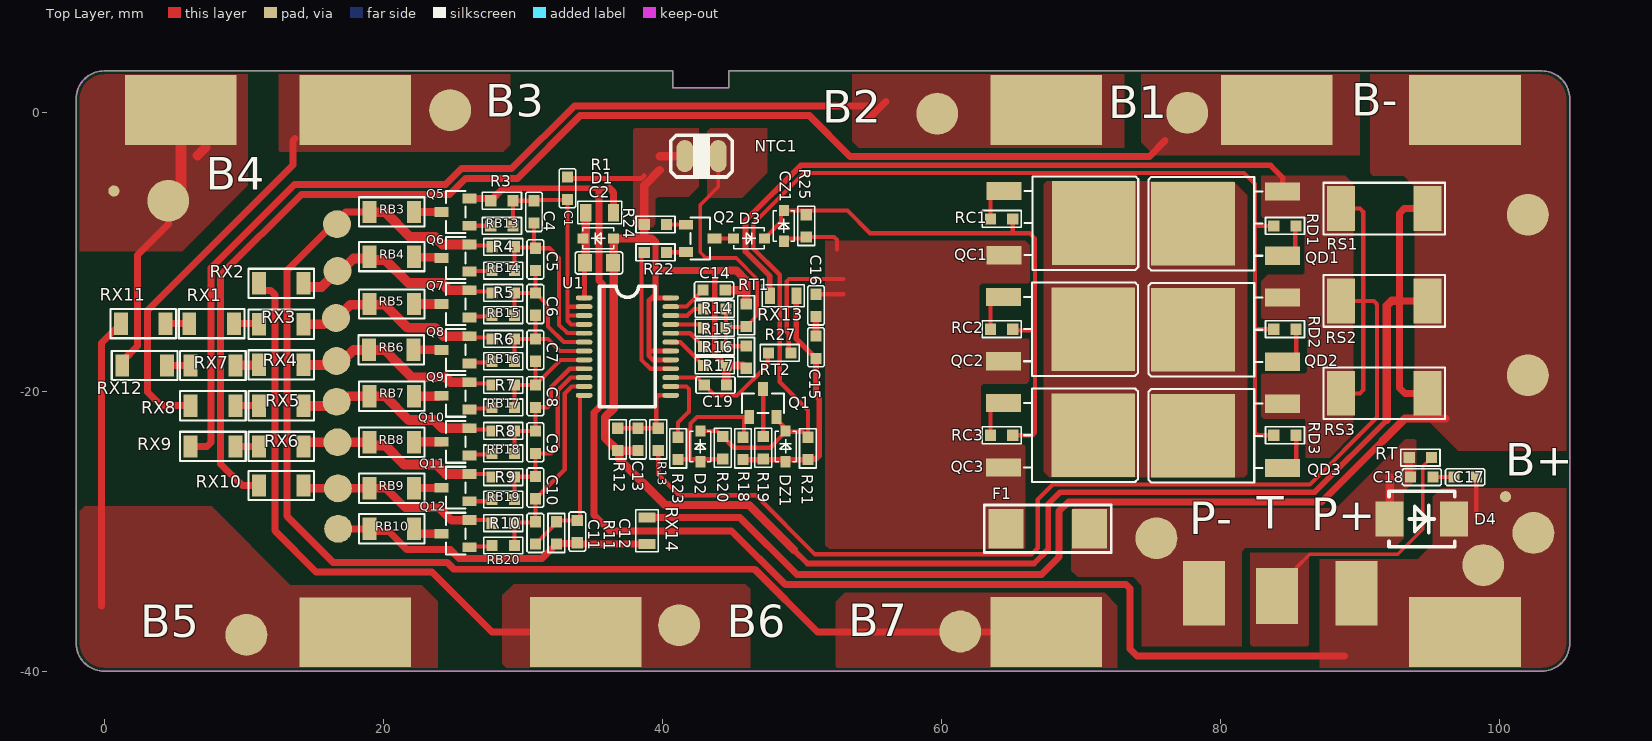
[diagram p0: Top Layer view]
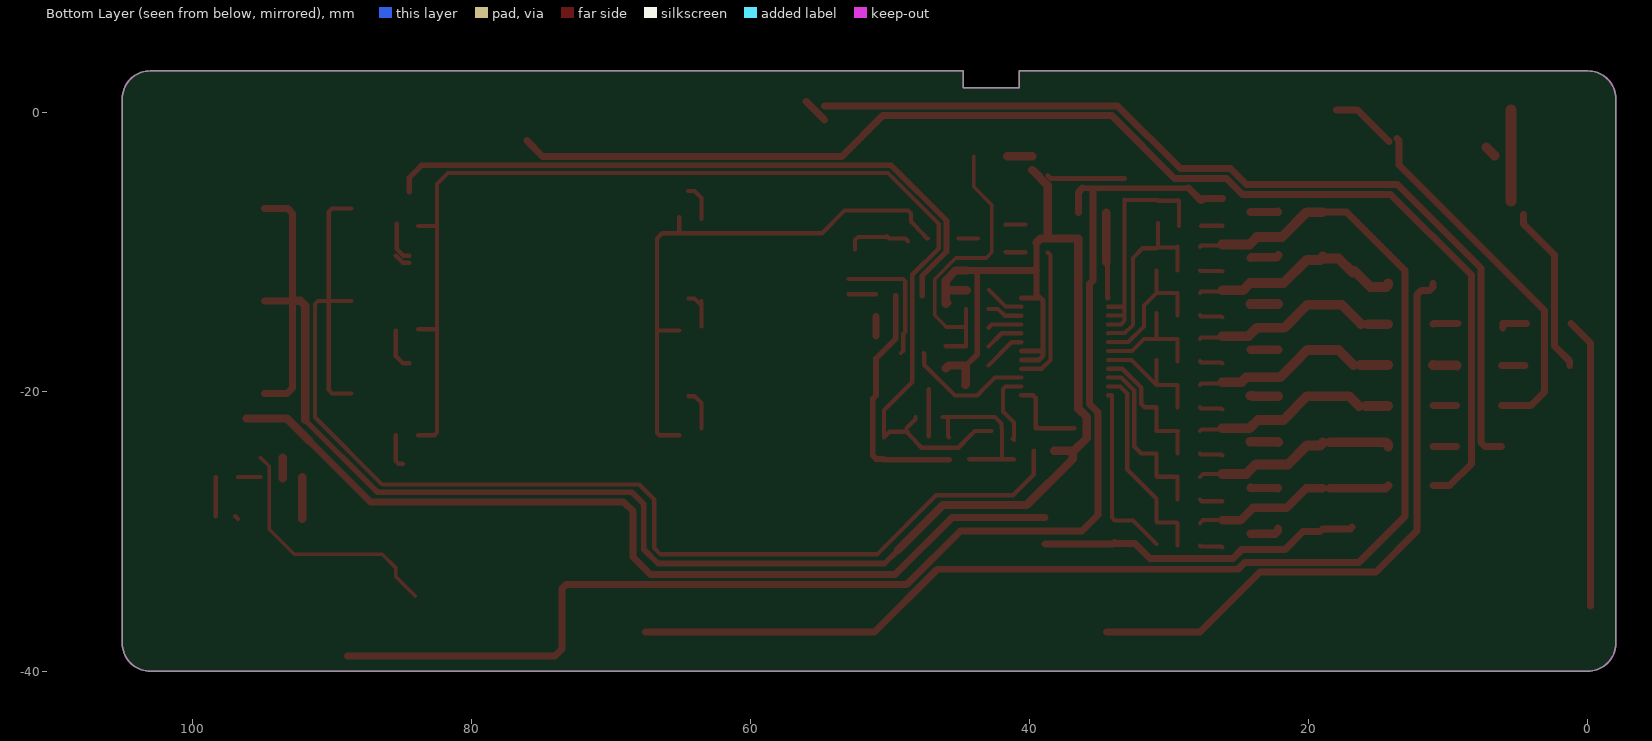
[diagram p1: Bottom Layer view, seen from below]
# Altium PCB MISC84401.PcbDoc
Units mm, origin at the board's own origin, x right, y up, seen from the top; angles counter-clockwise.
Board outline 107 x 43 mm, 2 copper layers (Top Layer, Bottom Layer); 122 components, 65 nets, 298 pads, 0 vias.
Unrouted connection lines stored in the file: 14.

## Layer stack, top to bottom (the 12.6 mil dielectric is the usual default, probably not edited)
Top Solder: solder mask 0.0102, Solder Resist, Dk 3.5
Top Layer: signal copper 0.0356
Dielectric 1: dielectric 0.32, FR-4, Dk 4.8
Bottom Layer: signal copper 0.0356
Bottom Solder: solder mask 0.0102, Solder Resist, Dk 3.5

## Board outline
-2,-38 -2,1 cw(c0,1) 0,3 40.751,3 40.751,1.8 44.751,1.8 44.751,3 103.001,3 cw(c103.001,1) 105.001,1 105.001,-38 cw(c103.001,-38) 103.001,-40 0,-40 cw(c0,-38)
board region "Default Layer Stack Region": -2,-38 -2,1 -2,1.197 -1.923,1.583 -1.772,1.947 -1.554,2.275 -1.275,2.554 -0.947,2.772 -0.583,2.923 -0.197,3 0,3 40.751,3 40.751,1.8 44.751,1.8 44.751,3 103.001,3 103.198,3 103.585,2.923 103.949,2.772 104.276,2.553 104.555,2.275 104.774,1.947 104.924,1.583 105.001,1.197 105.001,1 105.001,-38 105.001,-38.197 104.924,-38.584 104.774,-38.948 104.555,-39.275 104.276,-39.554 103.949,-39.773 103.585,-39.924 103.198,-40 103.001,-40 0,-40 -0.197,-40 -0.583,-39.924 -0.947,-39.773 -1.275,-39.554 -1.554,-39.275 -1.772,-38.948 -1.923,-38.584 -2,-38.197
board region "Layer Stack Region 1": -2,-38 -2,1 -2,1.197 -1.923,1.583 -1.772,1.947 -1.554,2.275 -1.275,2.554 -0.947,2.772 -0.583,2.923 -0.197,3 0,3 40.751,3 40.751,1.8 44.751,1.8 44.751,3 103.001,3 103.198,3 103.585,2.923 103.949,2.772 104.276,2.554 104.555,2.275 104.774,1.947 104.924,1.583 105.001,1.197 105.001,1 105.001,-38 105.001,-38.197 104.924,-38.584 104.774,-38.948 104.555,-39.275 104.276,-39.554 103.949,-39.773 103.585,-39.924 103.198,-40 103.001,-40 0,-40 -0.197,-40 -0.583,-39.924 -0.947,-39.773 -1.275,-39.554 -1.554,-39.275 -1.772,-38.948 -1.923,-38.584 -2,-38.197

## Design rules (kind name [scope] priority, off if disabled: settings)
Clearance [All] p1: gap=0.2 ignorepadtopadclearanceinfootprint=FALSE
ComponentClearance [All] p1: gap=0 collisioncheckmode=3 verticalgap=0 showdistances=FALSE
HoleToHoleClearance [All] p1: gap=0 allowstackedmicrovias=TRUE
MinimumSolderMaskSliver [All] p1: minsoldermaskwidth=0
PlaneConnect [All] p1: planeconnectstyle=Direct reliefexpansion=0.508 reliefentries=4 reliefconductorwidth=0.254 reliefairgap=0.254
PolygonConnect [All] p1: connectstyle=Direct reliefconductorwidth=0.254 reliefentries=4 polygonreliefangle="90 Angle" airgapwidth=0.254
RoutingVias [All] p1: holewidth=0.4 width=0.6 viastyle="Through Hole" minholewidth=0.4 minwidth=0.6 maxholewidth=0.4 maxwidth=0.6
SilkToSilkClearance [All] p1: silktosilkclearance=0
SilkToSolderMaskClearance [IsPad] p1: minsilkscreentomaskgap=0 clearancetoexposedcopper=TRUE
SolderMaskExpansion [All] p1: expansion=0.102 istentingtop=FALSE
SupplyNets "Schematic Supply Nets_1" [InNet('B-')] p1: voltage=0.000
SupplyNets "Schematic Supply Nets" [InNet('P-')] p2: voltage=0.000
Width [All] p1: maxlimit=1 minlimit=0.254 preferedwidth=0.254 minimp=50.000000 maximp=50.000000 favimp=50.000000
24 further rules are at their usual default settings.

## Components (designator, comment, footprint, x,y, rotation, side; value= is the part's Value field where it differs from the comment)
B1 "Pad" Pad10X8mm#1 84.001,0.2 r270 top locked
B2 "Pad" Pad10X8mm#2 67.501,-0.5 r270 top locked
B3 "Pad" Pad10X8mm#1 18,0.206 r270 top locked
B4 "Pad" Pad10X8mm#3 5.5,0.2 r270 top locked
B5 "Pad" Pad10X8mm#1 18,-37.2 r270 top locked
B6 "Pad" Pad10X8mm#3 34.5,-37.2 r270 top locked
B7 "Pad" Pad10X8mm#1 67.501,-37.194 r270 top locked
B+ "Pad" Pad10X8mm#1 97.501,-37.194 r270 top locked
B- "Pad" Pad10X8mm#3 97.501,0.2 r90 top locked
C1 "0.1uF" C0603A 33.2,-5.4 r270 top
C2 "1uF50V/0805" C0805A 35.45,-10.75 r180 top
C4 "0.1uF" C0603A 30.8,-7.1 r90 top
C5 "0.1uF" C0603A 30.9,-10.5 r90 top
C6 "0.1uF" C0603A 30.9,-13.7 r90 top
C7 "0.1uF" C0603A 30.9,-17 r90 top
C8 "0.1uF" C0603A 30.9,-20.3 r90 top
C9 "0.1uF" C0603A 30.9,-23.6 r90 top
C10 "0.1uF" C0603A 30.9,-26.85 r90 top
C11 "0.1uF" C0603A 30.9,-30.1 r90 top
C12 "1uF/NC*" C0603A 33.9,-30 r90 top
C13 "0.1uF" C0603A 38.25,-23.4 r90 top
C14 "0.1uF/NC*" C0603A 43.7,-12.7 r180 top
C15 "0.1uF" C0603A 51,-16.8 r270 top
C16 "0.1uF" C0603A 51,-13.8 r270 top
C17 "0.1uF" C0603A 97.5,-26.1 r0 top
C18 "0.1uF" C0603A 94.4,-26.1 r0 top
C19 "0.01uF/NC*" C0603A 43.8,-19.5 r0 top
CZ1 "15V" SOD323 48.7,-8.1 r270 top
D1 "56V" SOD323 35.4,-9 r0 top
D2 "1N4148SW/NC*" SOD323 42.72,-23.9 r270 top
D3 "1N4148SW" SOD323 46.2,-9 r180 top
D4 "RS3M" SMB(DO-214AA) 94.4,-29.1 r180 top
DZ1 "15V" SOD323 48.82,-23.9 r270 top
F1 "F2410 60V30A" F2410 67.6,-29.8 r0 top
NTC1 "10K B=3435" RT2.3X1.2-2 42.8,-3.1 r180 top
P+ "Pad" Pad10X8mm#4 82.122,-35.576 r270 top locked (schematic designator P+1)
P- "Pad" Pad10X8mm#5 86.327,-35.576 r270 top locked
Q1 "MMBT5401/N*" SOT23-3 47.2,-20.8 r0 top
Q2 "MMBT5401" SOT23-3 42.7,-9 r270 top
Q5 "MMBT5401" SOT23-3 25.189,-7.109 r90 top
Q6 "MMBT5401" SOT23-3 25.189,-10.401 r90 top
Q7 "MMBT5401" SOT23-3 25.189,-13.692 r90 top
Q8 "MMBT5401" SOT23-3 25.189,-16.984 r90 top
Q9 "MMBT5401" SOT23-3 25.189,-20.275 r90 top
Q10 "MMBT5401" SOT23-3 25.189,-23.567 r90 top
Q11 "MMBT5401" SOT23-3 25.189,-26.858 r90 top
Q12 "MMBT5401" SOT23-3 25.189,-30.15 r90 top
QC1 "TO-252 N MOS*" TO-252 67.687,-7.9 r270 top
QC2 "TO-252 N MOS*" TO-252 67.656,-15.5 r270 top
QC3 "TO-252 N MOS*" TO-252 67.656,-23.1 r270 top
QD1 "TO-252 N MOS*" TO-252 81.219,-7.939 r90 top
QD2 "TO-252 N MOS*" TO-252 81.219,-15.539 r90 top
QD3 "TO-252 N MOS*" TO-252 81.219,-23.139 r90 top
R1 "100R/1K*0805" R0805A#1 35.5,-7.15 r180 top
R3 "1K" R0603A 28.5,-6.3 r0 top
R4 "1K" R0603A 28.6,-9.6 r0 top
R5 "1K" R0603A 28.6,-12.9 r0 top
R6 "1K" R0603A 28.6,-16.2 r0 top
R7 "1K" R0603A 28.6,-19.5 r0 top
R8 "1K" R0603A 28.589,-22.792 r0 top
R9 "1K" R0603A 28.6,-26.1 r0 top
R10 "1K" R0603A 28.6,-29.4 r0 top
R11 "1K" R0603A 32.4,-30.1 r90 top
R12 "1K" R0603A 36.8,-23.4 r90 top
R13 "1K" R0603A 39.7,-23.4 r270 top
R14 "1K" R0603A 43.75,-14.05 r0 top
R15 "1K" R0603A 43.75,-15.4 r0 top
R16 "1K" R0603A 43.75,-16.75 r0 top
R17 "1K" R0603A 43.75,-18.1 r0 top
R18 "1K" R0603A 45.77,-24.042 r270 top
R19 "1K" R0603A 47.22,-24 r270 top
R20 "1K" R0603A 44.32,-24 r90 top
R21 "1K" R0603A 50.42,-24.042 r270 top
R22 "1K" R0603A 39.5,-10 r0 top
R23 "1K" R0603A 41.12,-24.042 r270 top
R24 "1K" R0603A 39.5,-8 r180 top
R25 "1K" R0603A 50.3,-8.1 r270 top
R27 "1K" R0603A 48.4,-17.2 r180 top
RB3 "51R" R1206A 20.6,-7.1 r0 top
RB4 "51R" R1206A 20.6,-10.3 r0 top
RB5 "51R" R1206A 20.6,-13.7 r0 top
RB6 "51R" R1206A 20.573,-16.984 r0 top
RB7 "51R" R1206A 20.6,-20.3 r0 top
RB8 "51R" R1206A 20.6,-23.6 r0 top
RB9 "51R" R1206A 20.6,-26.9 r0 top
RB10 "51R" R1206A 20.6,-29.8 r0 top
RB13 "1K" R0603A 28.5,-8.1 r0 top
RB14 "1K" R0603A 28.6,-11.3 r0 top
RB15 "1K" R0603A 28.6,-14.5 r0 top
RB16 "1K" R0603A 28.6,-17.8 r0 top
RB17 "1K" R0603A 28.6,-21.1 r0 top
RB18 "1K" R0603A 28.6,-24.4 r0 top
RB19 "1K" R0603A 28.6,-27.7 r0 top
RB20 "1K" R0603A 28.6,-31 r0 top
RC1 "1K" R0603A 64.3,-7.6 r0 top
RC2 "1K" R0603A 64.3,-15.5 r180 top
RC3 "1K" R0603A 64.3,-23.1 r180 top
RD1 "1K" R0603A 84.6,-8.1 r180 top
RD2 "1K" R0603A 84.6,-15.5 r180 top
RD3 "1K" R0603A 84.6,-23.1 r180 top
RS1 "R010" R2512L 91.7,-6.859 r180 top
RS2 "R010" R2512L 91.7,-13.48 r180 top
RS3 "R010" R2512L 91.7,-20.1 r180 top
RT "1K" R0603A 94.3,-24.7 r0 top
RT1 "1K" R0603A 46,-14.5 r90 top
RT2 "1K" R0603A 46,-17.5 r270 top
RX1 "1K" R1206A 7.7,-15.1 r180 top
RX2 "1K" R1206A 12.7,-12.22 r180 top
RX3 "1K" R1206A 12.7,-15.14 r180 top
RX4 "1K" R1206A 12.7,-18.06 r180 top
RX5 "1K" R1206A 12.7,-20.98 r180 top
RX6 "1K" R1206A 12.7,-23.9 r180 top
RX7 "1K" R1206A 7.8,-18.1 r180 top
RX8 "1K" R1206A 7.8,-20.98 r0 top
RX9 "1K" R1206A 7.8,-23.9 r0 top
RX10 "1K" R1206A 12.7,-26.7 r0 top
RX11 "1K" R1206A 2.8,-15.1 r180 top
RX12 "1K" R1206A 2.9,-18.1 r180 top
RX13 "1K" R0805A#2 48.65,-13.1 r180 top
RX14 "1K" R0805A#2 38.9,-29.95 r90 top
T "Pad" Pad10X8mm#6 84.019,-34.617 r90 top locked
U1 "CW1104/ERP2018" TSSOP-24(pin间距0.635mm) 37.491,-16.746 r0 top

## Footprints (in the part's own frame and the unit in brackets; to place one, negate y for a bottom-side part, rotate by r counter-clockwise, add the part's x,y. Pads: shape width x height; smd on the part's side, far side on the other; paste and mask are expansions set on the pad)
C0603A [mm] "贴片电容"
  rect 0.8x0.8 smd mask+0.08: 1(-0.8,0) 2(0.8,0)
  silkscreen extent -1.4,-0.6 1.4,0.6
C0805A [mm] "贴片电容"
  rect 1x1.25 smd: 1(-1,0)
  rect 1x1.25 smd mask+0.102: 2(1,0)
  silkscreen extent -1.7,-0.8 1.7,0.8
F2410 [mm] "贴片保险丝"
  rect 2.5x2.8 smd: 1(-3,0) 2(3,0)
  silkscreen extent -4.55,-1.7 4.55,1.7
Pad10X8mm#1 [mm]
  rect 5x8 smd: 1(0.006,0)
Pad10X8mm#2 [mm]
  rect 5x8 smd: 1(-0.7,0)
Pad10X8mm#3 [mm]
  rect 5x8 smd: 1(0,0)
Pad10X8mm#4 [mm]
  rect 4.6x3 smd: 1(-1.154,7.6)
Pad10X8mm#5 [mm]
  rect 4.6x3 smd: 1(-1.154,-7.524)
Pad10X8mm#6 [mm]
  rect 4x3 smd: 1(0,0)
R0603A [mm] "贴片电阻"
  rect 0.8x0.8 smd mask+0.08: 1(-0.8,0) 2(0.8,0)
  silkscreen extent -1.4,-0.6 1.4,0.6
R0805A#1 [mm] "贴片电阻"
  rect 0.8x1.25 smd paste+0 mask+0.08: 1(-1,0) 2(1,0)
  silkscreen extent -1.58,-0.8 1.58,0.8
R0805A#2 [mm] "贴片电阻"
  rect 0.7x1.2 smd paste+0 mask+0.08: 1(-0.95,0) 2(0.95,0)
  silkscreen extent -1.5,-0.8 1.5,0.8
R1206A [mm] "贴片电阻"
  rect 1x1.6 smd: 1(-1.6,0) 2(1.6,0)
  silkscreen extent -2.35,-1.05 2.35,1.05
R2512L [mm] "贴片电阻"
  rect 2x3.2 smd: 1(-3.1,0) 2(3.1,0)
  silkscreen extent -4.35,-1.85 4.35,1.85
RT2.3X1.2-2 [mm] "焊线NTC"
  oval 1.2x2.3 smd: 1(-1.2,0) 2(1.2,0)
  silkscreen extent -2.2,-1.55 2.2,1.5
SMB(DO-214AA) [mm] "贴片二极管"
  rect 2x2.5 smd: 1(-2.3,0) 2(2.3,0)
  silkscreen extent -2.35,-2 2.35,2
SOD323 [mm] "贴片二极管"
  rect 0.8x0.7 smd: 1(-1.1,0) 2(1.1,0)
  silkscreen extent -1.1,-0.75 1.1,0.75
SOT23-3 [mm] "贴片IC/MOS*"
  rect 0.7x1 smd: 1(-0.975,-1) 2(0.975,-1) 3(0,1.016)
  silkscreen extent -1.5,-0.7 1.5,0.7
TO-252 [mm]
  rect 1.3x2.5 smd: 1(-2.3,-3.212) 2(2.3,-3.212)
  rect 6x6 smd: 3(0,3.213)
  silkscreen extent -3.35,-1.75 3.35,6.4
TSSOP-24(pin间距0.635mm) [mm] "贴片IC"
  oval 1.2x0.35 smd: 1(-3.1,3.492) 1(-3.1,3.492) 2(-3.1,2.857) 3(-3.1,2.222) 4(-3.1,1.587) 5(-3.1,0.953) 6(-3.1,0.318) 7(-3.1,-0.318) 8(-3.1,-0.953) 9(-3.1,-1.587) 10(-3.1,-2.222) 11(-3.1,-2.858) 12(-3.1,-3.493) 13(3.1,-3.493) 13(3.1,-3.493) 14(3.1,-2.858) 15(3.1,-2.222) 16(3.1,-1.587) 17(3.1,-0.953) 18(3.1,-0.318) 19(3.1,0.318) 20(3.1,0.953) 21(3.1,1.587) 22(3.1,2.222) 23(3.1,2.857) 24(3.1,3.492)
  silkscreen extent -2,-4.33 2,4.33

## Part data
B1 B2 B3 B4 B5 B6 B7 B+ B- P+ P- T: "Connection pad (non-through-hole)"
C1 C2 C4 C5 C6 C7 C8 C9 C10 C11 C12 C13 C14 C15 C16 C17 C18 C19: library part CAP, "SMD capacitor"
CZ1 D1 DZ1: library part 5V6, "SMD Zener diode"
D2: library part 1N4148SW, "SMD diode"
D3 D4: "SMD diode"
F1: library part FUSE
NTC1: library part NTC, "SMD thermistor"
Q1: library part MMBT5401, "SMD transistor"
Q2 Q5 Q6 Q7 Q8 Q9 Q10 Q11 Q12: "SMD transistor"
QC1 QC2 QC3 QD1 QD2 QD3: library part "N MOS*", "SMD MOS"
R1 R3 R4 R5 R6 R7 R8 R9 R10 R11 R12 R13 R14 R15 R16 R17 R18 R19 R20 R21 R22 R23 R24 R25 R27 RB13 RB14 RB15 RB16 RB17 RB18 RB19 RB20 RC1 RC2 RC3 RD1 RD2 RD3 RT RT1 RT2 RX1 RX2 RX3 RX4 RX5 RX6 RX7 RX8 RX9 RX10 RX11 RX12 RX13 RX14: library part RES, "SMD resistor"
RB3 RB4 RB5 RB6 RB7 RB8 RB9 RB10: library part RES3, "Alloy SMD resistor"
RS1 RS2 RS3: library part RES2, "SMD alloy resistor"
U1: library part CW1104*, "Cellwise 7-10S battery protection IC"

## Free pads (board coordinates)
  round 0.8 smd: 2(0.7,-5.6) 2(100.4,-27.5)
  round 3 smd: 3(102,-18.8) 4(102,-7.3) 5(10.2,-37.4) 5(24.789,0.191) 5(59.689,-0.059) 5(61.339,-37.159) 5(77.6,0) 6(4.6,-6.3) 7(41.189,-36.709) 8(75.39,-30.48) 8(98.8,-32.4) 8(102.4,-30.1)
  rect 2.5x20 on Top Solder: 9(53.8,-20.7) 9(56.5,-20.7) 9(59.2,-20.7) 9(98.3,-13.8)
  round 2 smd: 10(16.61,-14.7) 10(16.64,-17.78) 10(16.66,-20.7) 10(16.69,-7.98) 10(16.72,-11.33) 10(16.75,-26.9) 10(16.77,-29.8) 11(16.725,-23.6)

## Nets (pads, with @x,y where several pads share a name; then routed paths per layer and width w, separated by ;. In a path a pad name is that pad's centre, name@x,y a point inside that pad or via, vN(x,y) a via of type N, cw(c..) or ccw(c..) an arc to the next point about the centre after c; other vN are vias at no path point)
B1: B1.1 pad.5@77.6,0 pad.10@16.75,-26.9 Q12.2 R10.1 RB9.1 RX10.1 RX10.2 | length 105.1
  Top Layer w0.3: Q12.2 27.575,-29.175 R10.1
  Top Layer w0.5: RX10.1 9.9,-26.7 8.35,-25.15 8.35,-11.63 14.138,-5.842 24.758,-5.842 25.9,-4.7 29.61,-4.7 34.11,-0.2 50.52,-0.2 53.44,-3.12 74.89,-3.12 76.02,-1.99
  Top Layer w0.6: RX10.2 14.5,-26.9 RB9.1@18.5,-26.9 ; RB9.1 20.193,-26.9 21.593,-28.3 24,-28.3 24.9,-29.2 26.164,-29.2 Q12.2
B2: B2.1 pad.5@59.689,-0.059 pad.11 Q11.2 R9.1 RB8.1 RX6.1 RX6.2 RX9.1 RX9.2 | length 83.8
  Top Layer w0.3: Q11.2 27.583,-25.883 R9.1
  Top Layer w0.5: RX9.1 7.357,-23.9 7.65,-23.607 7.65,-11.13 13.638,-5.142 24.458,-5.142 25.6,-4 29.2,-4 33.7,0.5 54.7,0.5 ; RX9.2 RX6.2 ; 54.7,-0.5 56,0.8
  Top Layer w0.7: RX6.1 14.3,-23.75 14.45,-23.6 RB8.1@18.5,-23.6 ; RB8.1 19,-23.69 19.15,-23.84 20.14,-23.84 21.5,-25.2 23.8,-25.2 24.483,-25.883 Q11.2
B3: B3.1 pad.5@24.789,0.191 pad.10@16.66,-20.7 Q10.2 R8.1 RB7.1 RX5.1 RX5.2 RX8.1 RX8.2 | length 46.7
  Top Layer w0.3: Q10.2 26.289,-22.692 27.689,-22.692 R8.1
  Top Layer w0.5: RX8.1 4.08,-20.98 3.1,-20 3.1,-14.173 13.537,-3.737 13.537,-1.983 13.68,-1.84 ; RX8.2 RX5.2 ; B3.1@14.25,-2.05 16.5,0.2 B3.1
  Top Layer w0.7: RX5.1 14.32,-21 pad.10@15.9,-21 ; pad.10@16.4,-21 17.1,-20.3 RB7.1 20.122,-20.3 21.822,-22 23.634,-22 24.226,-22.592 Q10.2
B4: B4.1 pad.2@0.7,-5.6 pad.6 pad.10@16.64,-17.78 Q9.2 R7.1 RB6.1 RX4.1 RX4.2 RX7.1 RX7.2 RX12.1 RX12.2 | length 37.4
  Top Layer w0.3: Q9.2 26.288,-19.4 27.7,-19.4 R7.1
  Top Layer w0.5: RX12.2 1.3,-17.8 2.4,-16.7 2.4,-10.176 4.6,-7.976 pad.6@4.6,-7.3 ; RX12.1 RX7.2
  Top Layer w0.7: 6.7,-3.05 7.279,-2.471 ; RX7.1 9.42,-18.08 11.08,-18.08 RX4.2 ; RX4.1 pad.10@16.3,-18.06 ; pad.10@16.8,-18.06 17.858,-17.002 20.113,-17.002 20.984,-17.873 22.061,-18.95 24.475,-18.95 24.825,-19.3 Q9.2
  Top Layer w0.8: pad.6@5.5,-6.3 B4.1
B5: B5.1 pad.5@10.2,-37.4 pad.10@16.61,-14.7 Q8.2 R6.1 RB5.1 RX1.1 RX1.2 RX3.1 RX3.2 RX11.1 RX11.2 | length 39.2
  Top Layer w0.3: Q8.2@26.18,-16 Q8.2 26.284,-16.104 27.704,-16.104 R6.1
  Top Layer w0.5: -0.2,-35.34 -0.2,-16.54 ; -0.2,-16.5 RX11.2 ; RX11.1 RX1.2 RX1.2@6.1,-15.4 ; RX1.1 11.06,-15.1 RX3.2
  Top Layer w0.7: RX3.1 pad.10@15.76,-15.14 ; pad.10@16.26,-15.14 17.651,-13.749 20.1,-13.749 21.751,-15.4 23.702,-15.4 24.302,-16 Q8.2@26.18,-16
B6: B6.1 pad.7 pad.10@16.72,-11.33 Q7.2 R5.1 RB4.1 RX2.1 RX2.2 | length 59.4
  Top Layer w0.3: Q7.2 26.28,-12.809 27.709,-12.809 R5.1
  Top Layer w0.5: RX2.2 11.1,-12.494 11.35,-12.744 11.937,-12.744 12.23,-13.036 12.23,-29.94 15.19,-32.9 23.5,-32.9 27.8,-37.2 B6.1
  Top Layer w0.7: RX2.1 14.3,-12.33 14.45,-12.48 15.57,-12.48 pad.10@16.72,-11.33 ; pad.10@16.845,-11.455 17.86,-10.44 18.86,-10.44 RB4.1 19,-10.39 19.15,-10.54 20.14,-10.54 21.8,-12.2 24.2,-12.2 24.717,-12.717 Q7.2
B7: B7.1 pad.5@61.339,-37.159 pad.10@16.69,-7.98 Q6.2 R4.1 RB3.1 | length 92.9
  Top Layer w0.3: Q6.2 26.276,-9.513 27.713,-9.513 R4.1
  Top Layer w0.5: RB3.1@19,-7.118 17.282,-7.118 13.1,-11.3 13.1,-28.9 16.4,-32.2 24.569,-32.2 25.069,-32.7 46.61,-32.7 51.11,-37.2 61.339,-37.2 B7.1
  Top Layer w0.7: RB3.1@19,-7.118 20.14,-7.118 21.922,-8.9 23.718,-8.9 24.243,-9.426 Q6.2
B+: B+.1 C17.2 D4.1 P+.1 pad.2@100.4,-27.5 pad.8@98.8,-32.4 pad.8@102.4,-30.1 Q5.2 R1.1 R3.1 | length 99.6
  Top Layer w0.3: D4.1 D4.1@96.9,-28.9 ; 98.3,-28.899 C17.2
  Top Layer w0.4: 28.6,-5.4 36.207,-5.4
  Top Layer w0.5: Q5.2 27.534,-6.134 R3.1 28.6,-5.4 ; 35.45,-5.45 35.45,-12 35.7,-12.25 35.7,-20.869 35.1,-21.469 35.1,-28.8 36.25,-29.95 44.96,-29.95 48.8,-33.79 73.207,-33.79 73.5,-34.083 73.5,-38.4 74,-38.9 88.872,-38.9 ; 36.207,-5.4 36.5,-5.693 R1.1
B-: B-.1 C1.1 C2.1 C12.1 C13.1 C14.1 C19.2 D1.2 NTC1.2 pad.3 pad.4 pad.10@16.77,-29.8 R11.1 R12.1 R17.2 R24.2 RB10.1 RS1.1 RS2.1 RS3.1 RT1.2 RT2.2 RX14.1 RX14.2 U1.17 U1.18 U1.24 | length 247.9
  Top Layer w0.35: C1.1@33.2,-4.7 38.5,-4.7 38.7,-4.5 ; 39.025,-13.459 39.025,-17.1 ; 39.255,-13.254 U1.24 ; U1.17 39.324,-17.699 39.025,-17.4 39.025,-17.1 ; U1.18 39.061,-17.064 39.025,-17.1
  Top Layer w0.4: 39.05,-13.459 39.255,-13.254 39.5,-13.009 39.5,-11.3 39.5,-9.3 ; 43.712,-11.3 43.75,-11.338 43.75,-17.316 44.033,-17.599 44.049,-17.599 R17.2 ; 49.4,-31.3 50.39,-32.29 66.62,-32.29 67.64,-31.27 67.64,-28.02 68.48,-27.18 86.72,-27.18 91.9,-22
  Top Layer w0.5: pad.10@16.9,-29.68 17.02,-29.8 RB10.1 ; RB10.1@19.2,-30.007 20.4,-30.007 21.693,-31.3 24.8,-31.3 25.425,-31.925 31.375,-31.925 R11.1 32.45,-30.85 33.85,-30.85 C12.1 34,-30.9 RX14.1 ; RX14.2 45.54,-29 49.63,-33.09 67.16,-33.09 68.42,-31.83 68.42,-28.54 69.09,-27.87 87.23,-27.87 91.6,-23.5 ; 39.5,-11.3 43.712,-11.3 44.459,-11.3 ; RS3.1 93.193,-20.1 92.8,-19.707 92.8,-13.454 ; RS2.1 92.826,-13.48 92.8,-13.454 ; RS1.1 93.141,-6.859 92.8,-7.2 92.8,-13.454
  Top Layer w0.6: C13.1 R12.1 ; 39.5,-9.3 39.5,-9.293 39.207,-9 38.6,-9 ; 39.8,-4.1 38.7,-5.2 R24.2 38.7,-8.9 38.6,-9 ; 39.8,-3.1 NTC1.2 ; 44.459,-11.3 45.3,-11.3 46,-12 46,-12.8 ; C14.1 45.9,-12.7 46,-12.8 ; C19.2 44.575,-19.475 44.575,-18.125 R17.2 45.8,-18.1 RT2.2 ; RT1.2 45.9,-13.6 46,-13.6 46,-12.8 ; 49.4,-31.3 46.2,-28.1 40.2,-28.1 36.9,-24.8 36.9,-24.3 R12.1 ; 91.6,-23.5 93.2,-21.9 96.1,-21.9 ; 91.9,-22 91.9,-13.805 92.251,-13.454 92.8,-13.454 ; R12.1 35.9,-23.3 35.9,-21.8 36.5,-21.2 D1.2 38.6,-9
CO: R22.1 U1.16 | length 10.1
  Top Layer w0.3: R22.1 38.5,-10.2 38.5,-17.7 39.134,-18.334 U1.16
CS: C15.2 DZ1.2 QD1.2 QD2.2 QD3.2 R13.2 R18.2 R19.2 R21.2 RS1.2 RS2.2 RS3.2 RX13.1 RX13.2 | length 153.9
  Top Layer w0.3: R13.2 39.7,-25.9 41.2,-27.4 46.71,-27.4 50.94,-31.63 66.45,-31.63 66.89,-31.19 66.89,-27.7 67.96,-26.63 86.38,-26.63 91.2,-21.81 91.2,-13.714 90.966,-13.48 90.2,-13.48 ; RS3.2 89.966,-20.1 90.2,-19.866 90.2,-13.48 ; RS2.2 90.2,-13.48 ; RS1.2 89.966,-6.859 90.2,-7.093 90.2,-13.48
  Top Layer w0.4: R18.2 R21.2 50.462,-24.8 50.986,-24.8 51.22,-24.566 51.22,-20.485 51,-20.265 C15.2 49.6,-16.2 RX13.1 ; RX13.2 47.7,-11.7 45.95,-9.95 45.95,-7.727 49.907,-3.77 83.56,-3.77 84.431,-4.641 QD1.2
DO: R23.1 U1.14 | length 5.3
  Top Layer w0.3: U1.14 41.724,-19.604 41.9,-19.779 41.9,-21.41 41.12,-22.19 R23.1 ; R23.1@41.12,-23.442 R23.1@41.22,-23.342
NetC13_2: C13.2 R12.2 R13.1 U1.13 | length 6
  Top Layer w0.3: R12.2 C13.2 39.561,-22.6 39.561,-20.414 39.737,-20.239 U1.13@40.591,-20.239
NetC14_2: C14.2 U1.23 | length 2.8
  Top Layer w0.3: U1.23 40.601,-13.879 41.721,-13.879 C14.2
NetC15_1: C15.1 C16.2 | length 1.4
  Top Layer w0.5: C15.1 C16.2
NetC16_1: C16.1 CZ1.2 F1.1 QC1.2 QC2.2 QC3.2 R25.2 R27.1 | length 16
  Top Layer w0.3: CZ1.2 48.9,-9 50.05,-9 R25.2@50.225,-8.825 ; R27.1 49.05,-17.05 49.05,-15.85 48.9,-15.7 48.9,-12.076 49.076,-11.9 52.955,-11.9 ; R25.2 52.3,-8.9 52.5,-9.1 52.5,-9.8 ; C16.1 52.961,-13
NetC17_1: C17.1 C18.2 | length 1.6
  Top Layer w0.3: C18.2@95.1,-26.1 C17.1
NetCZ1_1: CZ1.1 D3.1 R25.1 RC1.2 RC2.1 RC3.1 | length 39.8
  Top Layer w0.3: D3.1 47.35,-9 47.55,-8.8 47.55,-8.75 48.5,-7.8 48.5,-7.2 CZ1.1 50.3,-7 53.25,-7 54.88,-8.63 65.1,-8.63 ; RC3.1@65.096,-23.1 66.524,-23.1 66.7,-22.924 66.7,-15.6 ; RC2.1@65.1,-15.6 66.7,-15.6 ; RC1.2@65.1,-7.481 65.1,-8.63 ; 65.1,-8.63 66.32,-8.63 66.7,-9.01 66.7,-15.6
NetD2_1: D2.1 DZ1.1 Q1.2 R20.2 R21.1 RD1.2 RD2.2 RD3.2 | length 86.5
  Top Layer w0.3: D2.1 43.92,-22.8 R20.2 45.112,-23.992 47.723,-23.992 48.172,-23.543 48.172,-23.498 48.732,-22.938 DZ1.1@48.732,-22.887 ; Q1.2 48.175,-21.95 DZ1.1@48.821,-22.596 ; DZ1.1 48.82,-22.85 50.028,-22.85 R21.1 50.42,-21.31 48.4,-19.29 48.4,-11.6 46.5,-9.7 46.5,-7.955 50.135,-4.32 81.67,-4.32 82.456,-5.106 82.456,-8.1 ; RD3.2 82.645,-23.1 82.456,-22.911 82.456,-15.5 ; RD2.2 82.456,-15.5 ; RD1.2 82.456,-8.1 ; 82.456,-15.5 82.456,-8.1
NetD2_2: D2.2 Q1.1 R18.1 R20.1 R23.2 | length 11.7
  Top Layer w0.3: R23.2 41.141,-24.821 41.97,-24.821 ; R20.1 44.299,-24.821 41.97,-24.821 ; R18.1 45.845,-23.167 45.845,-21.8 ; Q1.1 45.845,-21.8 ; 41.97,-24.821 41.97,-22.628 42.02,-22.578 42.02,-22.255 42.475,-21.8 45.845,-21.8
NetD3_2: D3.2 Q2.3 | length 1.4
  Top Layer w0.3: Q2.3 D3.2
NetNTC1_1: NTC1.1 R14.2 R15.2 R16.2 RT1.1 RT2.1 | length 21.7
  Top Layer w0.254: NTC1.1 44,-5.3 42.7,-6.6 42.7,-10 43.1,-10.4 45.287,-10.4 46.8,-11.913 46.8,-14.5 RT1.1
  Top Layer w0.3: R14.2 R15.2 ; RT2.1 45.975,-16.725 44.575,-16.725 R16.2 R15.2 ; RT1.1 45.95,-15.35 44.6,-15.35 R15.2
NetQ1_3: Q1.3 R19.1 | length 3.4
  Top Layer w0.3: R19.1 Q1.3@47.22,-19.804
NetQ2_1: Q2.1 R24.1 | length 1.4
  Top Layer w0.3: R24.1 40.313,-8.013 41.688,-8.013 Q2.1
NetQ2_2: Q2.2 R22.2 | length 1.4
  Top Layer w0.3: R22.2 40.313,-9.988 41.687,-9.988 Q2.2
NetQ5_1: Q5.1 RB13.1 | length 1.5
  Top Layer w0.3: Q5.1 26.197,-8.092 27.692,-8.092 RB13.1
NetQ5_3: Q5.3 RB3.2 | length 2
  Top Layer w0.6: RB3.2 22.205,-7.105 24.168,-7.105 Q5.3
NetQ6_1: Q6.1 RB14.1 | length 1.6
  Top Layer w0.3: Q6.1 26.226,-11.338 27.762,-11.338 RB14.1
NetQ6_3: Q6.3 RB4.2 | length 2.1
  Top Layer w0.6: RB4.2@22.173,-10.201 22.323,-10.351 24.123,-10.351 Q6.3
NetQ7_1: Q7.1 RB15.1 | length 1.7
  Top Layer w0.3: Q7.1 26.272,-14.584 27.716,-14.584 RB15.1
NetQ7_3: Q7.3 RB5.2 | length 2
  Top Layer w0.7: RB5.2 24.015,-13.7 24.023,-13.692 Q7.3
NetQ8_1: Q8.1 RB16.1 | length 1.7
  Top Layer w0.3: Q8.1 26.268,-17.879 27.721,-17.879 RB16.1
NetQ8_3: Q8.3 RB6.2 | length 2
  Top Layer w0.6: RB6.2 Q8.3
NetQ9_1: Q9.1 RB17.1 | length 1.7
  Top Layer w0.3: Q9.1 26.264,-21.175 27.725,-21.175 RB17.1
NetQ9_3: Q9.3 RB7.2 | length 2
  Top Layer w0.7: RB7.2 23.998,-20.3 24.023,-20.275 Q9.3
NetQ10_1: Q10.1 RB18.1 | length 1.7
  Top Layer w0.3: Q10.1 26.26,-24.471 27.729,-24.471 RB18.1
NetQ10_3: Q10.3 RB8.2 | length 2
  Top Layer w0.7: RB8.2 22.233,-23.567 Q10.3
NetQ11_1: Q11.1 RB19.1 | length 1.7
  Top Layer w0.3: Q11.1 27.667,-27.833 RB19.1
NetQ11_3: Q11.3 RB9.2 | length 2
  Top Layer w0.6: RB9.2 22.221,-26.879 24.152,-26.879 Q11.3
NetQ12_1: Q12.1 RB20.1 | length 1.7
  Top Layer w0.3: Q12.1 26.251,-31.063 27.737,-31.063 RB20.1
NetQ12_3: Q12.3 RB10.2 | length 2.2
  Top Layer w0.6: RB10.2 22.2,-29.95 22.4,-30.15 Q12.3
NetQC1_1: QC1.1 RC1.1 | length 2.7
  Top Layer w0.3: RC1.1 63.5,-6.1 64,-5.6 QC1.1
NetQC1_3: QC1.3 QC2.3 QC3.3 QD1.3 QD2.3 QD3.3
NetQC2_1: QC2.1 RC2.2 | length 3
  Top Layer w0.3: RC2.2@63.5,-15.3 QC2.1@63.5,-13.5 ; QC2.1@63.5,-13.8 64,-13.3 QC2.1@64.444,-13.3
NetQC3_1: QC3.1 RC3.2 | length 3
  Top Layer w0.3: 63.5,-22.6 63.5,-20.8 64,-20.3 QC3.1@64.444,-20.3
NetQD1_1: QD1.1 RD1.1 | length 4.1
  Top Layer w0.3: QD1.1@84.431,-10.739 84.9,-10.739 QD1.1@85.4,-10.239 ; QD1.1 84.84,-10.239 85.34,-9.739 RD1.1@85.34,-7.93
NetQD2_1: QD2.1 RD2.1 | length 3
  Top Layer w0.3: QD2.1@84.431,-17.939 84.9,-17.939 85.4,-17.439 RD2.1@85.4,-15.6
NetQD3_1: QD3.1 RD3.1 | length 2.4
  Top Layer w0.3: QD3.1@84.9,-25.139 85.2,-25.139 85.4,-24.939 RD3.1
NetR14_1: R14.1 U1.22 | length 2.6
  Top Layer w0.3: U1.22 40.601,-14.533 41.774,-14.533 42.257,-14.05 R14.1
NetR15_1: R15.1 U1.21 | length 2.5
  Top Layer w0.3: U1.21 42.709,-15.159 R15.1
NetR16_1: R16.1 U1.20 | length 2.8
  Top Layer w0.3: U1.20 41.994,-15.794 R16.1
NetR17_1: R17.1 U1.19 | length 3.1
  Top Layer w0.3: U1.19 40.601,-16.438 41.288,-16.438 R17.1
P-: C18.1 D4.2 F1.2 P-.1 pad.8@75.39,-30.48 RT.1 | length 4.5
  Top Layer w0.6: D4.2 92.1,-26.1 ; C18.1@93.5,-26.2 RT.1@93.5,-24.69
T: RT.2 T.1 | length 18.2
  Top Layer w0.254: T.1 85.392,-33.244 85.392,-32.608 86.385,-31.615 92.685,-31.615 94.473,-29.827 94.473,-25.327 RT.2
VC0: C11.1 C12.2 R11.2 U1.12 | length 13
  Top Layer w0.3: C11.1 32.6,-29.2 C12.2 34.1,-29 34.1,-20.262 34.123,-20.239 U1.12
VC1: C10.1 C11.2 R10.2 RB20.2 U1.11 | length 14.8
  Top Layer w0.3: RB20.2 R10.2 29.45,-29.35 30.85,-29.35 C11.2 C10.1 33,-25.55 33,-20.107 33.503,-19.604 U1.11
VC2: C9.1 C10.2 R9.2 RB19.2 U1.10 | length 12.9
  Top Layer w0.3: RB19.2 R9.2 29.425,-26.075 30.875,-26.075 C10.2 C9.1 32,-24.4 32.5,-23.9 32.5,-19.9 33.431,-18.969 U1.10
VC3: C8.1 C9.2 R8.2 RB18.2 U1.9 | length 10.1
  Top Layer w0.3: R8.2 R8.2@29.393,-22.796 ; RB18.2 29.394,-24.394 29.394,-22.798 R8.2@29.393,-22.796 ; U1.9 33.359,-18.334 32,-19.693 32,-20.85 31.75,-21.1 C8.1 C9.2 30.896,-22.796 R8.2@29.393,-22.796
VC4: C7.1 C8.2 R7.2 RB17.2 U1.8 | length 9.1
  Top Layer w0.3: RB17.2 R7.2 C8.2 ; C7.1@30.9,-17.7 C8.2 ; U1.8 32.701,-17.699 C8.2
VC5: C6.1 C7.2 R6.2 RB16.2 U1.7 | length 8.8
  Top Layer w0.3: RB16.2 R6.2 C7.2 31.8,-16.2 32.664,-17.064 U1.7 ; C7.2@30.85,-16.15 30.9,-16.1 C6.1@30.9,-14.35
VC6: C5.1 C6.2 R5.2 RB15.2 U1.6 | length 10.5
  Top Layer w0.3: RB15.2 R5.2 C6.2 ; C5.1 C6.2 ; U1.6 32.929,-16.429 31.8,-15.3 31.8,-13.8 C6.2
VC7: C4.1 C5.2 R4.2 RB14.2 U1.5 | length 13.9
  Top Layer w0.3: RB14.2 R4.2 29.45,-9.65 30.85,-9.65 C5.2 ; C4.1 30.8,-9.6 C5.2 ; U1.5 34.381,-15.784 33.184,-15.784 32.6,-15.2 32.6,-10.4 31.9,-9.7 C5.2
VC8: C1.2 C4.2 R3.2 RB13.2 U1.2 U1.3 U1.4 | length 18
  Top Layer w0.3: RB13.2 R3.2 C4.2 30.85,-6.25 33.15,-6.25 C1.2 33.2,-14.55 ; 33.374,-13.889 U1.2 ; U1.4 33.459,-15.159 33.301,-15.001 33.2,-14.9 33.2,-14.55 ; U1.3 33.226,-14.524 33.2,-14.55
VDD: C2.2 D1.1 R1.2 U1.1 | length 6.2
  Top Layer w0.35: U1.1@34.391,-13.254 34.42,-13.254 34.42,-10.78 C2.2 C2.2@34.5,-10.7
  Top Layer w0.6: C2.2@34.5,-10.7 R1.2
VM: C19.1 R27.2 U1.15 | length 9.3
  Top Layer w0.3: U1.15 42.469,-18.969 C19.1 43.75,-20.25 45.35,-20.25 47.545,-18.055 47.545,-17.255 R27.2

## Polygon pours and split planes (outlines as drawn)
B1 on Top Layer "NONET_L02_P-001" (solid, remove dead copper, pour order 12): 74.3,3.1 74.3,-2.1 75.25,-3.05 89.95,-3.05 89.95,4.35 88.6,3 74.2,3
P- on Top Layer "NONET_L02_P-001" (solid, remove dead copper, pour order 4): 81.755,-31.175 92.415,-31.175 93.1,-30.49 93.1,-27.15 94,-26.25 94,-23.5 93.9,-23.4 93.2,-23.4 88.28,-28.32 69.48,-28.32 69.3,-28.5 69.3,-32.79 69.75,-33.24 73.72,-33.24 74.35,-33.88 74.35,-38.21 81.5,-38.21 81.5,-31.43
B7 on Top Layer "NONET_L02_P-001" (solid, remove dead copper, pour order 10): 52.75,-40 52.41,-39.66 52.41,-35.03 53.05,-34.39 71.69,-34.39 72.6,-35.3 72.6,-40
B- on Top Layer "NONET_L02_P-001" (solid, remove dead copper, pour order 15): 37.9,-1.2 38,-1.1 42.6,-1.1 42.6,-5.3 41.9,-6 39.7,-6 39.5,-6.2 39.5,-8 39.3,-8.2 38,-8.2 37.9,-8.1
NetNTC1_1 on Top Layer "NONET_L02_P-001" (solid, remove dead copper, pour order 14): 43.3,-1.1 43.2,-1.2 43.2,-3.55 43.2,-6.1 45.7,-6.1 47.5,-4.3 47.5,-1.1
NetC16_1 on Top Layer "NONET_L02_P-001" (solid, remove dead copper, pour order 3): 51.95,-31.24 51.67,-30.97 51.67,-9.18 65.98,-9.18 66.3,-9.5 66.3,-12.1 66.2,-12.2 62.9,-12.2 62.7,-12.4 62.7,-16 62.9,-16.2 66.2,-16.2 66.288,-16.288 66.288,-19.212 66.1,-19.4 63,-19.4 62.8,-19.6 62.8,-23.6 62.9,-23.7 62.909,-23.691 65.788,-23.691 66,-23.903 66,-31.17 65.93,-31.24
B3 on Top Layer "NONET_L02_P-001" (solid, remove dead copper, pour order 6): 12.5,2.9 12.5,-2.7 12.6,-2.8 28.6,-2.8 29.1,-2.3 29.1,2.8 28.8,3.1 12.5,3.1 12.4,3
T on Top Layer "NONET_L02_P-001" (solid, remove dead copper, pour order 13): 86.3,-31.51 82.1,-31.51 82.1,-38.07 82.24,-38.21 86.2,-38.21 86.3,-38.11
B2 on Top Layer "NONET_L02_P-001" (solid, remove dead copper, pour order 11): 73.1,2.99 72.89,3.2 53.8,3.2 53.6,3 53.6,-2.02 54.08,-2.5 73.1,-2.5
NetQC1_3 on Top Layer "NONET_L02_P-001" (solid, remove dead copper, pour order 2): 67.3,-5.13 67.53,-4.9 80.89,-4.9 81.89,-5.9 81.9,-5.9 81.9,-25.88 81.67,-26.11 67.72,-26.11 67.31,-25.7 67.31,-25.51 67.3,-25.5
B6 on Top Layer "NONET_L02_P-001" (solid, remove dead copper, pour order 9): 29.08,-40 28.54,-39.46 28.54,-34.55 29.33,-33.76 45.95,-33.76 46.3,-34.11 46.3,-39.8 46.1,-40
B5 on Top Layer "NONET_L02_P-001" (solid, remove dead copper, pour order 8): 22.77,-33.85 23.9,-34.98 23.9,-39.9 -1.5,-39.9 -2,-39.4 -2,-28.8 -1.4,-28.2 7.7,-28.2 13.35,-33.85
B4 on Top Layer "NONET_L02_P-001" (solid, remove dead copper, pour order 7): -2,-9.7 -1.8,-9.9 5.6,-9.9 10.3,-5.2 10.3,3 -2,3
B+ on Top Layer "NONET_L02_P-001" (solid, remove dead copper, pour order 5): 94.1,-32 95.2,-30.9 95.2,-27.5 95.8,-26.9 105,-26.9 105,-39.1 104.1,-40 87.1,-40 87.1,-32
CS on Top Layer "NONET_L02_P-001" (solid, remove dead copper, pour order 1): 82.9,-7.377 83.023,-7.5 86,-7.5 86,-9.72 86,-11.47 85.881,-11.589 83.371,-11.589 82.9,-12.06 82.9,-14.65 83.01,-14.76 86.05,-14.76 86.2,-14.91 86.2,-18.52 86.031,-18.689 82.981,-18.689 82.9,-18.77 82.9,-21.74 83.07,-21.91 85.97,-21.91 86.1,-22.05 86.1,-24.7 87.8,-24.7 89.5,-23 89.5,-5.1 88.91,-4.51 82.9,-4.51
B- on Top Layer "NONET_L02_P-001" (solid, remove dead copper, pour order 0): 90.71,1.9 90.71,2.84 90.92,3.05 104.54,3.05 104.63,3.14 105.18,2.59 105.2,1.68 105.2,-23.9 104.9,-24.2 99.65,-24.2 97,-24.2 93.9,-21.1 93.9,-5.3 93.1,-4.5 90.9,-4.5 90.7,-4.3 90.7,1.9

## Keep-outs
Keep-Out Layer:
  the board outline again, w0.1

## Silkscreen, mask and mechanical layers (free items; w line width, h text height)
Mechanical 1:
  region: -7.643,1 -7.976,1 -7.809,2
  region: -7.809,-39 -7.976,-38 -7.643,-38
  region: 105.001,-47.003 104.001,-47.169 104.001,-46.836
  region: -1,-47.169 -2,-47.003 -1,-46.836
  lines w0.013: -8.309,-39 -0.25,-39 ; -8.309,2 -0.25,2 ; -7.809,-38 -7.809,1 ; -2,-47.503 -2,-39.25 ; -1,-47.003 104.001,-47.003 ; 0,-39 cw(c0,-37) -2,-37 -2,0 cw(c0,0) 0,2 103.001,2 cw(c103.001,0) 105.001,0 105.001,-37 cw(c103.001,-37) 103.001,-39 ; 0,-39 103.001,-39 ; 93.419,1.7 101.501,1.7 ; 105.001,-47.503 105.001,-37.25 ; 1.5,-3.3 9.5,-3.3 ; 1.5,-3.3 1.5,1.7 ; 1.5,-3.3 1.5,1.7 ; 1.5,-3.3 9.5,-3.3 ; 1.5,1.7 9.5,1.7 ; 1.5,1.7 9.5,1.7 ; 9.5,-3.3 9.5,1.7 ; 9.5,-3.3 9.5,1.7 ; 14,-38.7 14,-33.7 ; 14,-38.7 22,-38.7 ; 14,-38.7 14,-33.7 ; 14,-38.7 22,-38.7 ; 14,-33.7 22,-33.7 ; 14,-33.7 22,-33.7 ; 14,-3.3 14,1.7 ; 14,-3.3 22,-3.3 ; 14,-3.3 14,1.7 ; 14,-3.3 22,-3.3 ; 14,1.7 22,1.7 ; 14,1.7 22,1.7 ; 22,-38.7 22,-33.7 ; 22,-38.7 22,-33.7 ; 22,-3.3 22,1.7 ; 22,-3.3 22,1.7 ; 30.5,-38.7 38.5,-38.7 ; 30.5,-38.7 30.5,-33.7 ; 30.5,-38.7 30.5,-33.7 ; 30.5,-38.7 38.5,-38.7 ; 30.5,-33.7 38.5,-33.7 ; 30.5,-33.7 38.5,-33.7 ; 38.5,-38.7 38.5,-33.7 ; 38.5,-38.7 38.5,-33.7 ; 63.501,-38.7 71.501,-38.7 ; 63.501,-38.7 63.501,-33.7 ; 63.501,-38.7 63.501,-33.7 ; 63.501,-38.7 71.501,-38.7 ; 63.501,-33.7 71.501,-33.7 ; 63.501,-33.7 71.501,-33.7 ; 63.501,-3.3 63.501,1.7 ; 63.501,-3.3 71.501,-3.3 ; 63.501,-3.3 63.501,1.7 ; 63.501,-3.3 71.501,-3.3 ; 63.501,1.7 71.501,1.7 ; 63.501,1.7 71.501,1.7 ; 71.501,-38.7 71.501,-33.7 ; 71.501,-38.7 71.501,-33.7 ; 71.501,-3.3 71.501,1.7 ; 71.501,-3.3 71.501,1.7 ; 77.303,-34.739 77.303,-30.105 ; 77.303,-34.739 80.278,-34.739 ; 77.303,-34.739 77.303,-30.105 ; 77.303,-34.739 80.278,-34.739 ; 77.303,-30.105 80.278,-30.105 ; 77.303,-30.105 80.278,-30.105 ; 80.001,-3.3 80.001,1.7 ; 80.001,-3.3 88.001,-3.3 ; 80.001,-3.3 80.001,1.7 ; 80.001,-3.3 88.001,-3.3 ; 80.001,1.7 88.001,1.7 ; 80.001,1.7 88.001,1.7 ; 80.278,-34.739 80.278,-30.105 ; 80.278,-34.739 80.278,-30.105 ; 82.981,-34.739 82.981,-30.495 ; 82.981,-34.739 85.519,-34.739 ; 82.981,-34.739 82.981,-30.495 ; 82.981,-34.739 85.519,-34.739 ; 82.981,-30.495 85.519,-30.495 ; 82.981,-30.495 85.519,-30.495 ; 85.519,-34.739 85.519,-30.495 ; 85.519,-34.739 85.519,-30.495 ; 88.001,-3.3 88.001,1.7 ; 88.001,-3.3 88.001,1.7 ; 88.222,-34.739 88.222,-30.105 ; 88.222,-34.739 91.198,-34.739 ; 88.222,-34.739 88.222,-30.105 ; 88.222,-34.739 91.198,-34.739 ; 88.222,-30.105 91.198,-30.105 ; 88.222,-30.105 91.198,-30.105 ; 91.198,-34.739 91.198,-30.105 ; 91.198,-34.739 91.198,-30.105 ; 93.501,-38.7 101.501,-38.7 ; 93.501,-38.7 93.501,-33.7 ; 93.501,-38.7 93.501,-33.7 ; 93.501,-38.7 101.501,-38.7 ; 93.501,-33.7 101.501,-33.7 ; 93.501,-33.7 101.501,-33.7 ; 93.501,-3.3 93.501,1.7 ; 93.501,-3.3 101.501,-3.3 ; 93.501,-3.3 101.501,-3.3 ; 93.501,-3.3 93.501,1.7 ; 93.501,1.7 101.501,1.7 ; 101.501,-38.7 101.501,-33.7 ; 101.501,-38.7 101.501,-33.7 ; 101.501,-3.3 101.501,1.7 ; 101.501,-3.3 101.501,1.7
  text "B2" at 68.445,-3.856 h1.45 r180
  text "B-" at 98.257,-4.175 h1.45 r180
  text "B4" at 6.387,-4.386 h1.45 r180
  text "B1" at 83.793,-4.386 h1.45 r180
  text "B3" at 18.772,-5.581 h1.45 r180
  text "41.0004" at -11.049,-19 h1 r90
  text "T" at 85.358,-28.427 h1.16 r180
  text "P-" at 79.635,-28.496 h1.16 r180
  text "P+" at 90.659,-28.541 h1.16 r180
  text "B7" at 67.938,-31.069 h1.45 r180
  text "B6" at 35.304,-31.172 h1.45 r180
  text "B5" at 19.694,-31.376 h1.45 r180
  text "B+" at 98.257,-31.376 h1.45 r180
  text "107.0012" at 48.704,-46.742 h1